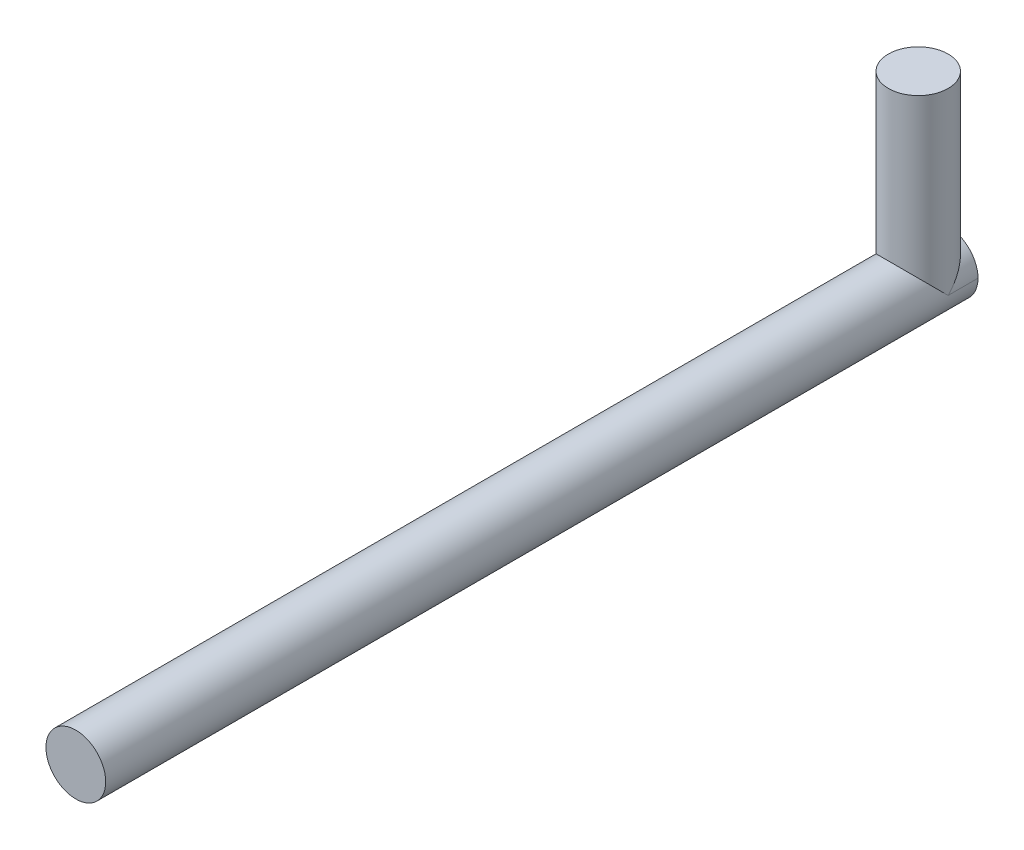
from build123d import *
from build123d.topology import SkipClean

# Parameters (mm, degrees)
SKETCH_1_R      = 2.5
EXTRUDE_1_DEPTH = 73
SKETCH_2_R      = 2.5
EXTRUDE_2_DEPTH = 15


with BuildPart() as part:
    # 草图1 → 凸台-拉伸1 (new body)
    with BuildSketch(Plane.XY):
        Circle(SKETCH_1_R)
    extrude(amount=EXTRUDE_1_DEPTH)

    # 草图2 → 凸台-拉伸2 (add)
    with SkipClean():  # the faces are left unmerged after this step: merging them gives an invalid solid
        with BuildSketch(Plane(origin=(0, 0, 0), x_dir=(1, 0, 0), z_dir=(0, 1, 0))):
            with Locations(Location((0, -2.5, 0), (0, 0, 90))):
                Circle(SKETCH_2_R)
        extrude(amount=EXTRUDE_2_DEPTH)


solid = part.part
